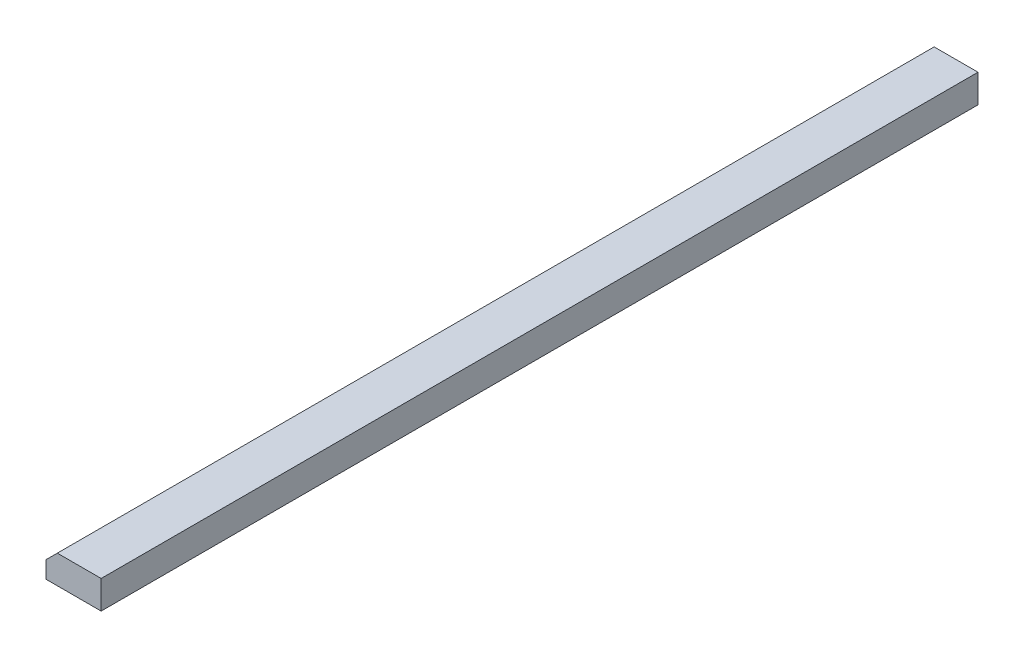
from build123d import *

# Parameters (mm, degrees)
SKETCH1_W           = 39
SKETCH1_H           = 20
BOSS_EXTRUDE1_DEPTH = 620
CHAMFER1_SIZE       = 8


with BuildPart() as part:
    # Sketch1 → Boss-Extrude1 (new body)
    with BuildSketch(Plane.XY):
        with Locations((19.5, 10)):
            Rectangle(SKETCH1_W, SKETCH1_H)
    extrude(amount=BOSS_EXTRUDE1_DEPTH)

    # Chamfer1
    chamfer1_edges = [part.edges().sort_by_distance(p)[0] for p in [
        (0, 20, 310),
    ]]
    chamfer(chamfer1_edges, length=CHAMFER1_SIZE)


solid = part.part
